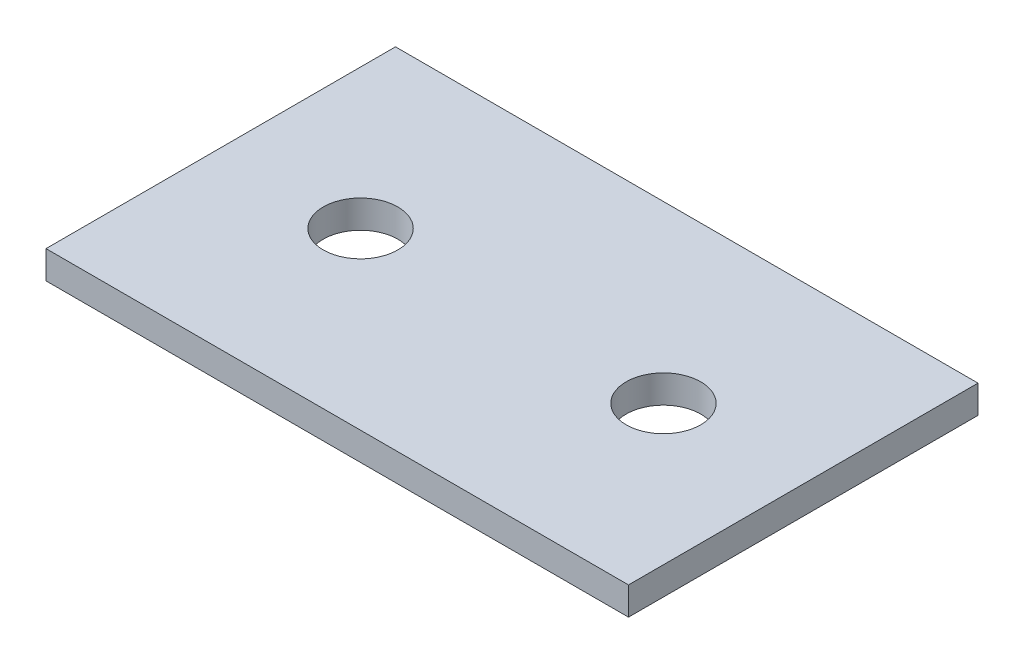
SolidWorks part; units mm, degrees
material "45"
ref_plane "前视基准面" through (0, 0, 0) normal (0, 0, 1) x (1, 0, 0)
ref_plane "上视基准面" through (0, 0, 0) normal (0, 1, 0) x (1, 0, 0)
ref_plane "右视基准面" through (0, 0, 0) normal (1, 0, 0) x (0, 0, -1)
sketch "草图1" plane through (0, 0, 0) normal (0, 1, 0) x (1, 0, 0)
  line L1 (-125, -75) -> (125, -75)
  line L2 (-125, -75) -> (-125, 75)
  line L3 (-125, 75) -> (125, 75)
  line L4 (125, -75) -> (125, 75)
  line L5 (-125, -75) -> (125, 75) construction
  line L6 (-125, 75) -> (125, -75) construction
  point P0 (0, 0)
  dimension "D1" = 250
  dimension "D2" = 150
extrude "凸台-拉伸1" add sketch "草图1" along normal blind 12
sketch "草图2" plane through (0, 0, 0) normal (0, -1, 0) x (-1, 0, 0)
  line L0 (-125, 75) -> (125, 75) construction
  line L1 (-125, -75) -> (-125, 75) construction
  line L2 (125, 75) -> (125, -75) construction
  line L3 (125, -75) -> (-125, -75) construction
  circle A0 centre (-108, 58) radius 10
  circle A1 centre (108, 58) radius 10
  circle A2 centre (-108, -58) radius 10
  circle A3 centre (108, -58) radius 10
extrude "切除-拉伸1" cut sketch "草图2" against normal blind 2
sketch "草图3" plane through (0, 12, 0) normal (0, 1, 0) x (1, 0, 0)
  circle A0 centre (-65, 0) radius 16
  circle A1 centre (65, 0) radius 16
extrude "切除-拉伸2" cut sketch "草图3" against normal up to next
equation "\"D3@草图2\"=\"D2@草图2\""
equation "\"D5@草图2\"=\"D4@草图2\""
equation "\"D6@草图2\"=\"D2@草图2\""
equation "\"D3@草图3\"=\"D2@草图3\""
